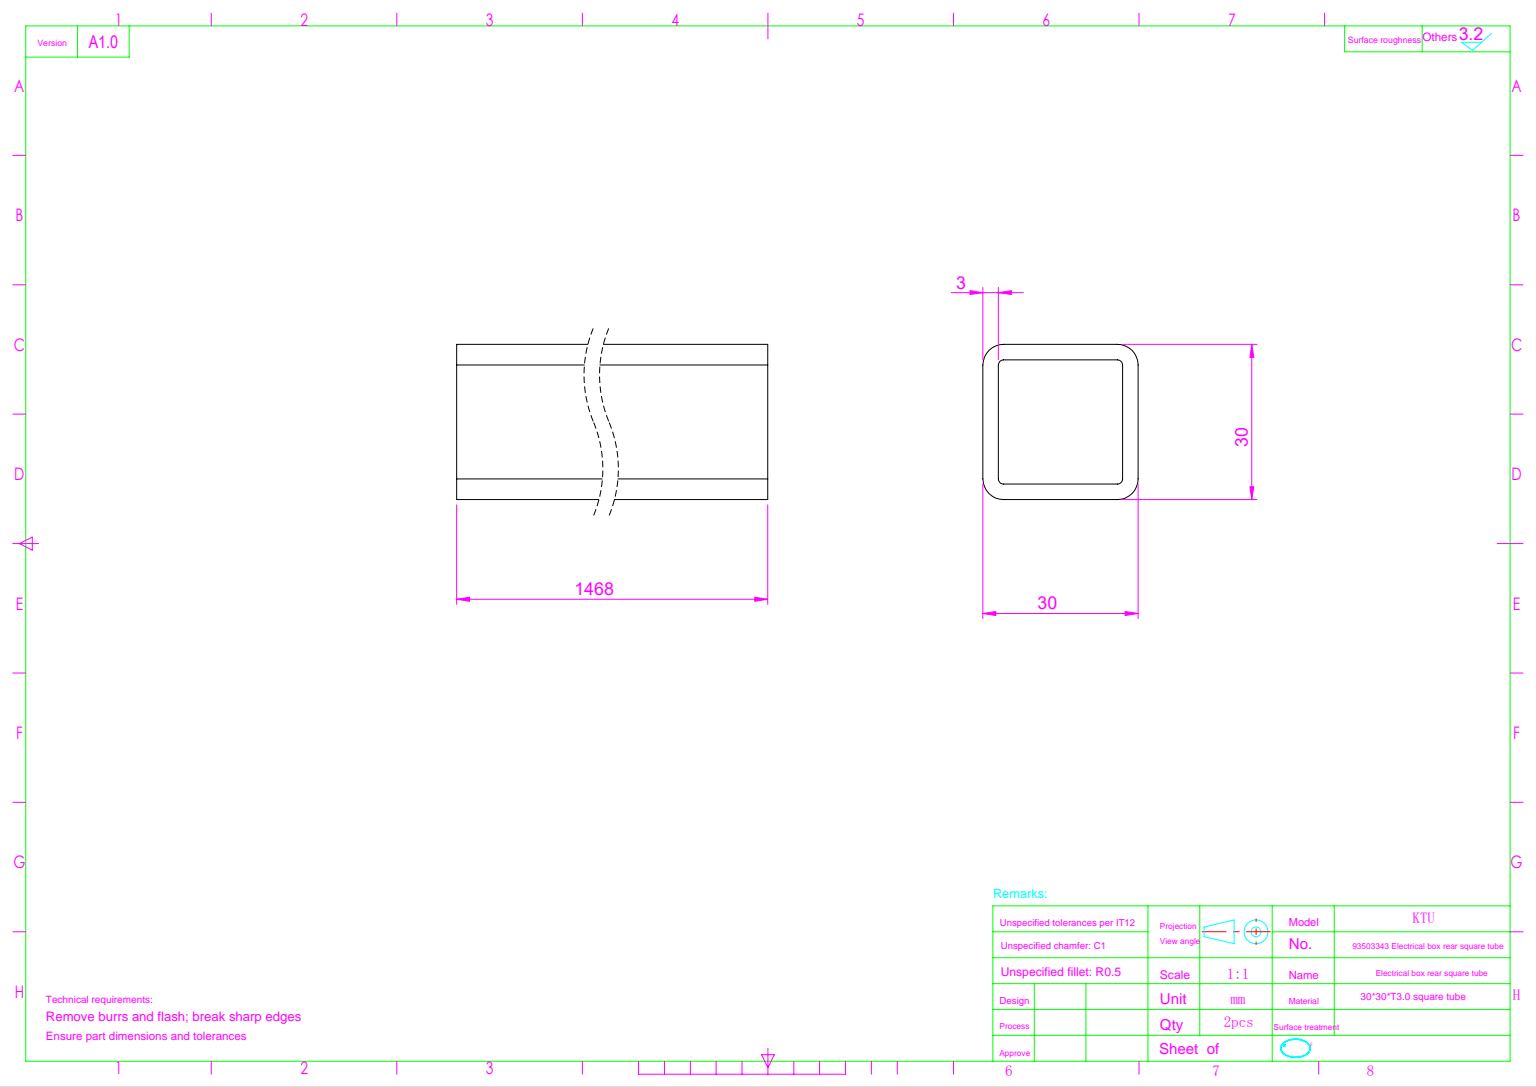
SolidWorks part; units mm, degrees
ref_plane "前视基准面" through (0, 0, 0) normal (0, 0, 1) x (1, 0, 0)
ref_plane "上视基准面" through (0, 0, 0) normal (0, 1, 0) x (1, 0, 0)
ref_plane "右视基准面" through (0, 0, 0) normal (1, 0, 0) x (0, 0, -1)
sketch "草图2" plane through (0, 0, 0) normal (0, 0, 1) x (1, 0, 0)
  line L1 (-11, 15) -> (11, 15)
  line L2 (-15, 11) -> (-15, -11)
  line L3 (-11, -15) -> (11, -15)
  line L4 (15, 11) -> (15, -11)
  line L5 (-15, 15) -> (15, -15) construction
  line L6 (-15, -15) -> (15, 15) construction
  arc A0 (11, 15) -> (15, 11) centre (11, 11) cw
  arc A1 (11, -15) -> (15, -11) centre (11, -11) ccw
  arc A2 (-15, -11) -> (-11, -15) centre (-11, -11) ccw
  arc A3 (-11, 15) -> (-15, 11) centre (-11, 11) ccw
  point P0 (0, 0)
  dimension "D3" = 4
  dimension "D1" = 30
  dimension "D2" = 30
extrude "拉伸-薄壁1" add sketch "草图2" along normal mid plane 1468 thin
